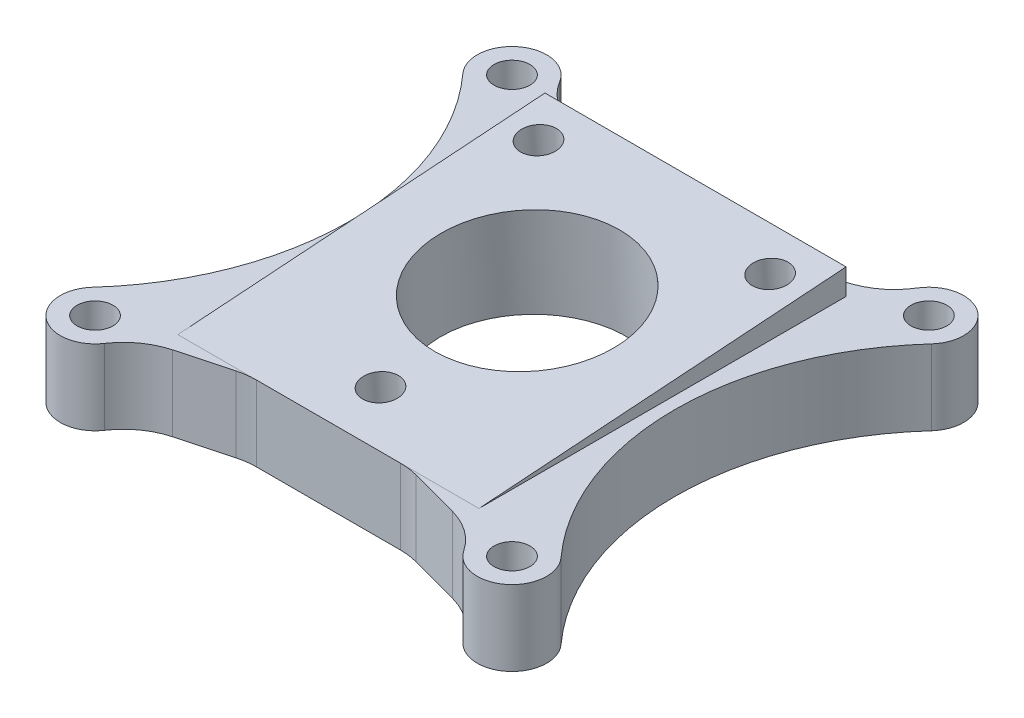
from build123d import *

# Parameters (mm, degrees)
SKETCH_1_R           = 1.55
EXTRUDE_1_DEPTH      = 6.5
EXTRUDE_2_DEPTH      = 13
EXTRUDE_2_DEPTH_BACK = 13
FILLET_1_R           = 6
SKETCH_5_R           = 1.55
SKETCH_5_R_2         = 8
CUT_EXTRUDE_3_DEPTH  = 32.013570632
SKETCH_6_R           = 3
CUT_EXTRUDE_10_DEPTH = 6


with BuildPart() as part:
    # 草图1 → 凸台-拉伸1 (new body)
    with BuildSketch(Plane(origin=(0, 0, 0), x_dir=(1, 0, 0), z_dir=(0, 1, 0))):
        with BuildLine():
            Line((-15, 18), (-9, 15.85))
            Line((-9, 15.85), (9, 15.85))
            Line((9, 15.85), (15, 18))
            ThreePointArc((15, 18), (19.079157226, 20.799181966), (20.223613121, 15.986161702))
            ThreePointArc((20.223613121, 15.986161702), (14.060533289, 0), (20.223613121, -15.986161702))
            ThreePointArc((20.223613121, -15.986161702), (19.079157226, -20.799181966), (15, -18))
            Line((15, -18), (7, -15.85))
            Line((7, -15.85), (-7, -15.85))
            Line((-7, -15.85), (-15, -18))
            ThreePointArc((-15, -18), (-19.079157226, -20.799181966), (-20.223613121, -15.986161702))
            ThreePointArc((-20.223613121, -15.986161702), (-14.060533289, 0), (-20.223613121, 15.986161702))
            ThreePointArc((-20.223613121, 15.986161702), (-19.079157226, 20.799181966), (-15, 18))
        make_face()
        with Locations(Location((18, 18, 0), (0, 0, 90))):
            Circle(SKETCH_1_R, mode=Mode.SUBTRACT)
        with Locations(Location((18, -18, 0), (0, 0, 90))):
            Circle(SKETCH_1_R, mode=Mode.SUBTRACT)
        with Locations(Location((-18, -18, 0), (0, 0, 90))):
            Circle(SKETCH_1_R, mode=Mode.SUBTRACT)
        with Locations(Location((-18, 18, 0), (0, 0, 90))):
            Circle(SKETCH_1_R, mode=Mode.SUBTRACT)
    extrude(amount=EXTRUDE_1_DEPTH)

    # 草图3 → 凸台-拉伸2 (add, two sides: drawn at the far end of the back side and taken through both)
    with BuildSketch(Plane(origin=(0, 0, 0), x_dir=(0, 0, -1), z_dir=(1, 0, 0)).offset(-EXTRUDE_2_DEPTH_BACK)):
        Polygon((-15.85, 6.5), (15.85, 6.5), (15.85, 8.716679939), align=None)
    extrude(amount=EXTRUDE_2_DEPTH + EXTRUDE_2_DEPTH_BACK)

    # 圆角1
    fillet_1_edges = [part.edges().sort_by_distance(p)[0] for p in [
        (15, 3.25, 18),
        (7, 3.25, 15.85),
        (-7, 3.25, 15.85),
        (-15, 3.25, 18),
        (-15, 3.25, -18),
        (-9, 3.25, -15.85),
        (9, 3.25, -15.85),
        (15, 3.25, -18),
    ]]
    fillet(fillet_1_edges, radius=FILLET_1_R)

    # 草图5 → 切除-拉伸3 (cut, through all)
    with BuildSketch(Plane(origin=(0, 7.571318049, 0.529438133), x_dir=(1, 0, 0), z_dir=(0, 0.9975640502598243, 0.06975647374412569))):
        with Locations(Location((10, 12.85, 0), (0, 0, 270))):
            Circle(SKETCH_5_R)
        with Locations(Location((0, -10.85, 0), (0, 0, 270))):
            Circle(SKETCH_5_R)
        with Locations(Location((-10, 12.85, 0), (0, 0, 270))):
            Circle(SKETCH_5_R)
        with Locations(Location((0, 1.85, 0), (0, 0, 270))):
            Circle(SKETCH_5_R_2)
    extrude(amount=-CUT_EXTRUDE_3_DEPTH, mode=Mode.SUBTRACT)

    # 草图6 → 切除-拉伸10 (cut)
    with BuildSketch(Plane(origin=(0, 1.528635135, -42.076453462), x_dir=(-1, 0, 0), z_dir=(0, 0.9975640502598243, 0.06975647374412568))):
        with Locations(Location((0, 52.930589533, 0), (0, 0, 270))):
            Circle(SKETCH_6_R)
        with Locations(Location((10, 29.230589533, 0), (0, 0, 270))):
            Circle(SKETCH_6_R)
        with Locations(Location((-10, 29.230589533, 0), (0, 0, 270))):
            Circle(SKETCH_6_R)
    extrude(amount=CUT_EXTRUDE_10_DEPTH, mode=Mode.SUBTRACT)


solid = part.part
